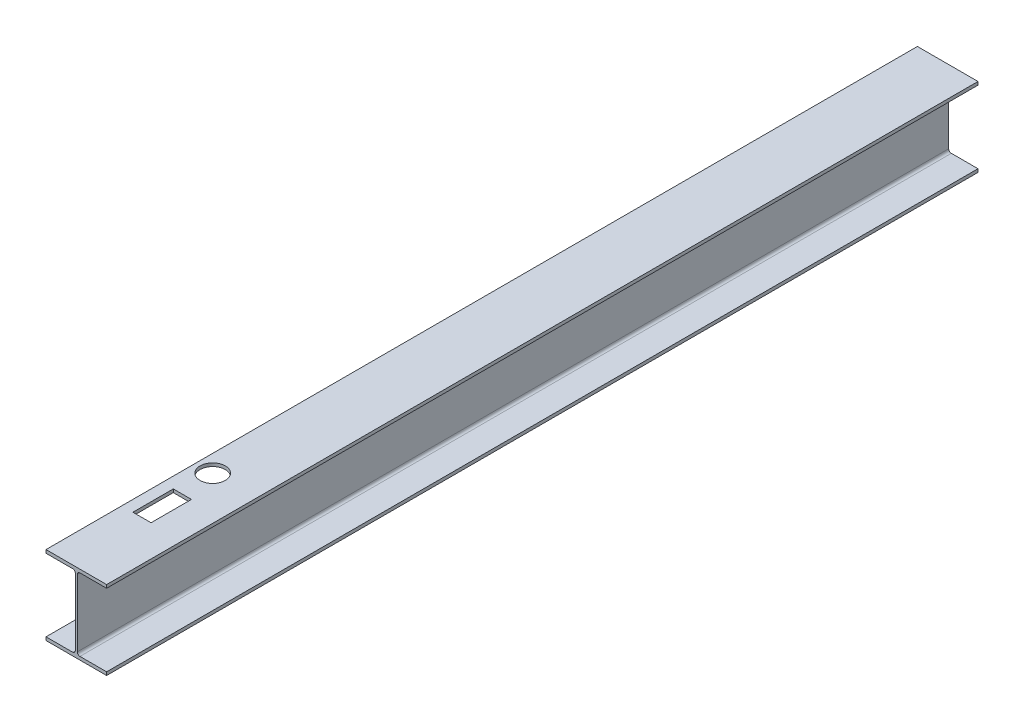
from build123d import *

# Parameters (mm, degrees)
BOSS_EXTRUDE1_DEPTH = 4313
SKETCH2_R           = 62.5
SKETCH2_W           = 90
SKETCH2_H           = 200
CUT_EXTRUDE1_DEPTH  = 30
CUT_EXTRUDE2_REACH  = 4335.37
SKETCH3_R           = 25.5


with BuildPart() as part:
    # Sketch1 → Boss-Extrude1 (new body)
    with BuildSketch(Plane.XY):
        with BuildLine():
            Line((0, 0), (300, 0))
            Line((300, 0), (300, 16))
            Line((300, 16), (168, 16))
            ThreePointArc((168, 16), (158.807611845, 19.807611845), (155, 29))
            Line((155, 29), (155, 361))
            ThreePointArc((155, 361), (158.807611845, 370.192388155), (168, 374))
            Line((168, 374), (300, 374))
            Line((300, 374), (300, 390))
            Line((300, 390), (0, 390))
            Line((0, 390), (0, 374))
            Line((0, 374), (132, 374))
            ThreePointArc((132, 374), (141.192388155, 370.192388155), (145, 361))
            Line((145, 361), (145, 29))
            ThreePointArc((145, 29), (141.192388155, 19.807611845), (132, 16))
            Line((132, 16), (0, 16))
            Line((0, 16), (0, 0))
        make_face()
    extrude(amount=BOSS_EXTRUDE1_DEPTH)

    # Sketch2 → Cut-Extrude1 (cut)
    with BuildSketch(Plane(origin=(0, 390, 0), x_dir=(1, 0, 0), z_dir=(0, 1, 0))):
        with Locations(Location((85, -3573, 0), (0, 0, 270))):
            Circle(SKETCH2_R)
        with Locations((100, -3838)):
            Rectangle(SKETCH2_W, SKETCH2_H)
    extrude(amount=-CUT_EXTRUDE1_DEPTH, mode=Mode.SUBTRACT)

    # Sketch3 → Cut-Extrude2 (cut, up to next)
    with BuildSketch(Plane.ZY.offset(-145), mode=Mode.PRIVATE) as cut_extrude2_sk1:
        with Locations(Location((3838, 315, 0), (0, 0, 270))):
            Circle(SKETCH3_R)
    cut_extrude2_tool1 = extrude(cut_extrude2_sk1.sketch, amount=-CUT_EXTRUDE2_REACH, mode=Mode.PRIVATE) & part.part
    add(cut_extrude2_tool1.solids().sort_by_distance((145, 315, 3838))[0], mode=Mode.SUBTRACT)


solid = part.part
